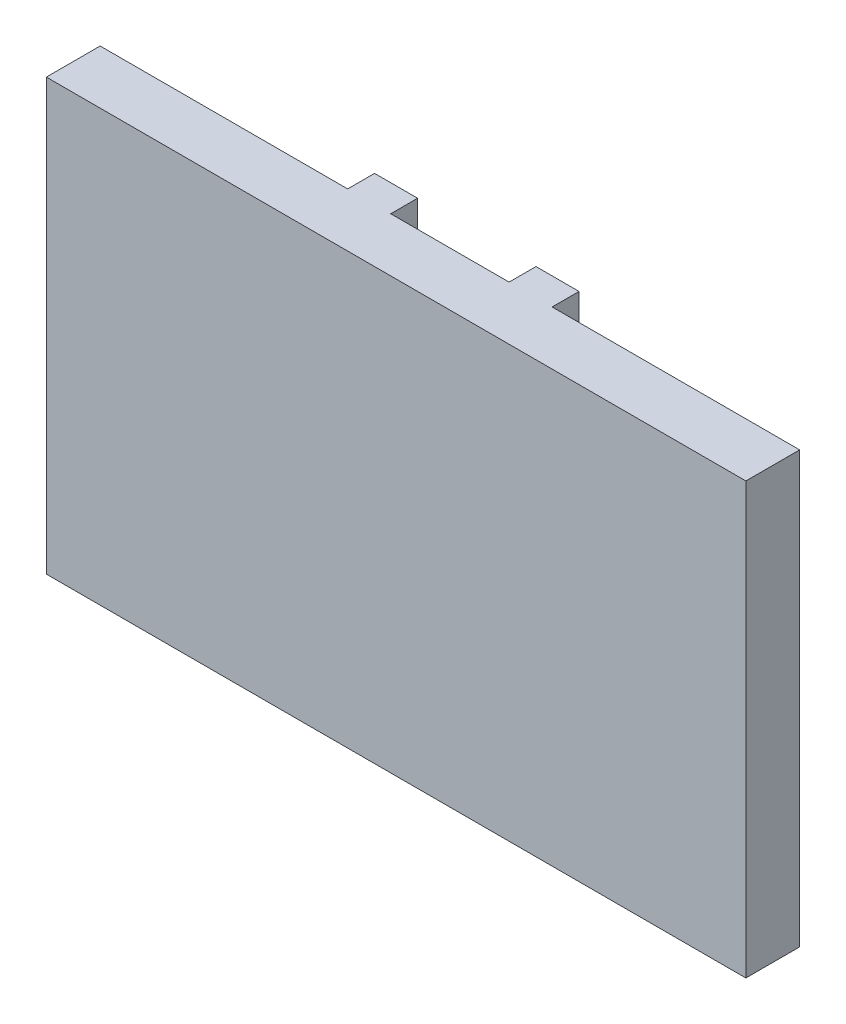
from build123d import *

# Parameters (mm, degrees)
SKETCH3_W           = 130
SKETCH3_H           = 80
BOSS_EXTRUDE1_DEPTH = 10
SKETCH4_W           = 8
SKETCH4_H           = 80
BOSS_EXTRUDE2_DEPTH = 5


with BuildPart() as part:
    # Sketch3 → Boss-Extrude1 (new body)
    with BuildSketch(Plane.XY):
        with Locations((720, 119)):
            Rectangle(SKETCH3_W, SKETCH3_H)
    extrude(amount=BOSS_EXTRUDE1_DEPTH)

    # Sketch4 → Boss-Extrude2 (add)
    with BuildSketch(Plane(origin=(0, 0, 0), x_dir=(-1, 0, 0), z_dir=(0, 0, -1))):
        with Locations((-735, 119)):
            Rectangle(SKETCH4_W, SKETCH4_H)
        with Locations((-705, 119)):
            Rectangle(SKETCH4_W, SKETCH4_H)
    extrude(amount=BOSS_EXTRUDE2_DEPTH)


solid = part.part
